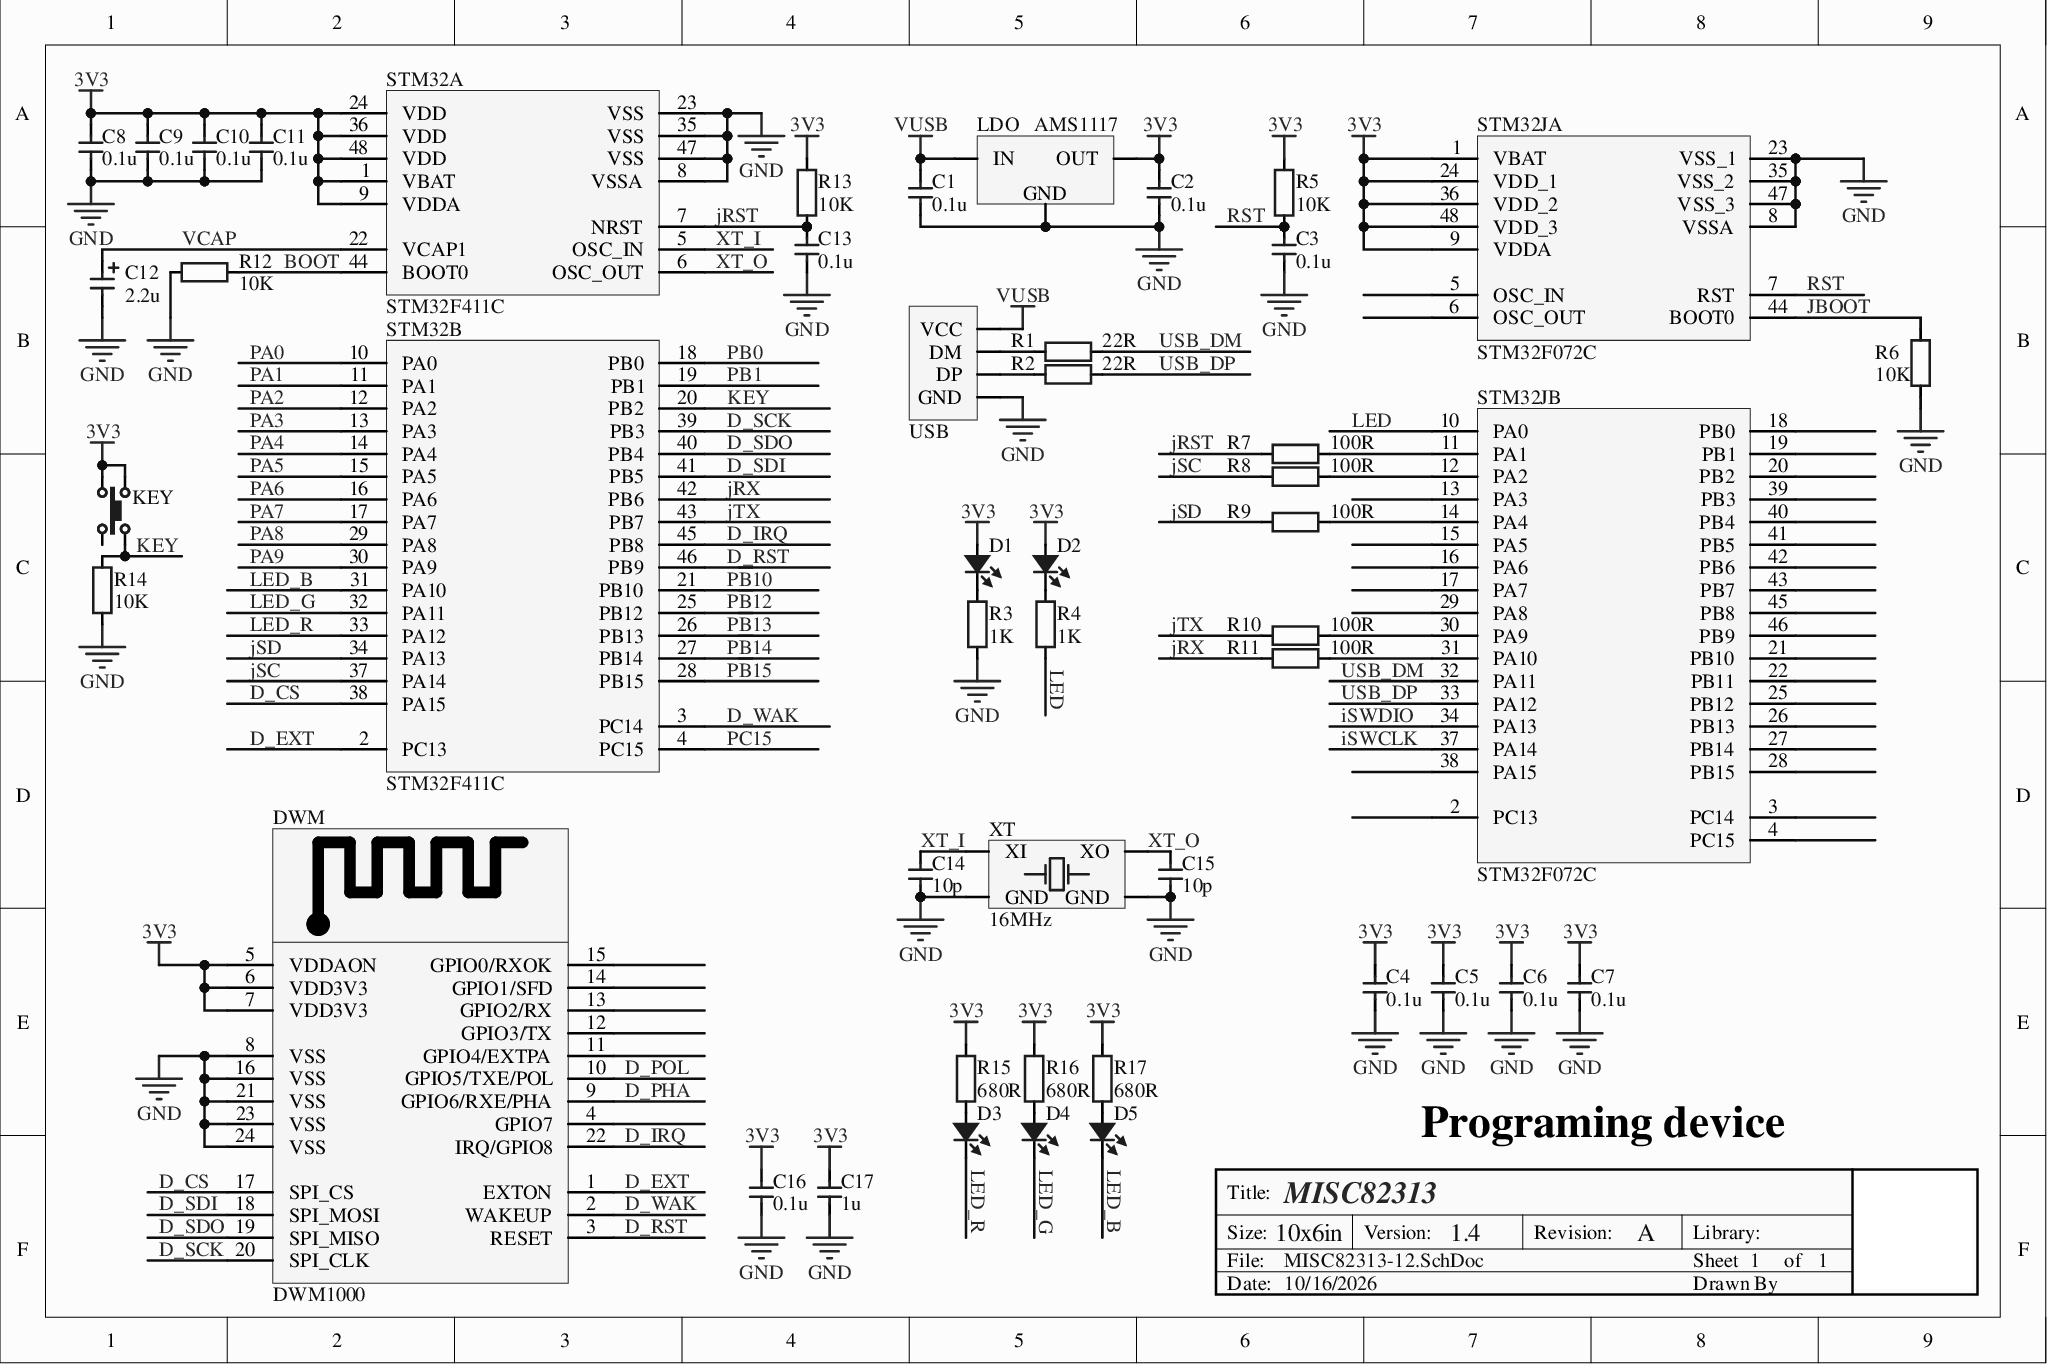
[diagram p0: MISC82313-12.SchDoc]
# Altium project MISC82313-6.PrjPCB
1 sheet, 46 parts. Net scope: global (net labels, ports and power ports of the same name join across sheets).
Board file: MISC82313-9.PcbDoc

## Sheet MISC82313-12.SchDoc: MISC82313
size 228 x 152 mm; Revision: A; SheetNumber: 1; SheetTotal: 1; Version: 1.4

### Parts
C1  value 0.1u  [CAP_0603]  (hidden comment: Cap_0603)
C2  value 0.1u  [CAP_0603]  (hidden comment: Cap_0603)
C3  value 0.1u  [CAP_0603]  (hidden comment: Cap_0603)
C4  value 0.1u  [CAP_0603]  (hidden comment: Cap_0603)
C5  value 0.1u  [CAP_0603]  (hidden comment: Cap_0603)
C6  value 0.1u  [CAP_0603]  (hidden comment: Cap_0603)
C7  value 0.1u  [CAP_0603]  (hidden comment: Cap_0603)
C8  value 0.1u  [CAP_0603]  (hidden comment: Cap_0603)
C9  value 0.1u  [CAP_0603]  (hidden comment: Cap_0603)
C10  value 0.1u  [CAP_0603]  (hidden comment: Cap_0603)
C11  value 0.1u  [CAP_0603]  (hidden comment: Cap_0603)
C12  value 2.2u  [CAP_TAN_P0805]  (hidden comment: Cap_Tan_0805)
C13  value 0.1u  [CAP_0603]  (hidden comment: Cap_0603)
C14  value 10p  [CAP_0603]  (hidden comment: Cap_0603)
C15  value 10p  [CAP_0603]  (hidden comment: Cap_0603)
C16  value 0.1u  [CAP_0603]  (hidden comment: Cap_0603)
C17  value 1u  [CAP_0603]  (hidden comment: Cap_0603)
D1  LED_0603  [LED_0603_YELLOW]  (value not drawn)
D2  LED_0603  [LED_0603_ORANGE]  (value not drawn)
D3  LED_0603  [LED_0603_RED]  (value not drawn)
D4  LED_0603  [LED_0603_GREEN]  (value not drawn)
D5  LED_0603  [LED_0603_BLUE]  (value not drawn)
DWM  DWM1000  [DWM1000]
KEY  ButtonTACT  [ButtonTACT_3.5*3.55_90]  (value not drawn)
LDO  AMS1117  [SOT89-3]
R1  value 22R  [RES_0603]  (hidden comment: Res_0603)
R2  value 22R  [RES_0603]  (hidden comment: Res_0603)
R3  value 1K  [RES_0603]  (hidden comment: Res_0603)
R4  value 1K  [RES_0603]  (hidden comment: Res_0603)
R5  value 10K  [RES_0603]  (hidden comment: Res_0603)
R6  value 10K  [RES_0603]  (hidden comment: Res_0603)
R7  value 100R  [RES_0603]  (hidden comment: Res_0603)
R8  value 100R  [RES_0603]  (hidden comment: Res_0603)
R9  value 100R  [RES_0603]  (hidden comment: Res_0603)
R10  value 100R  [RES_0603]  (hidden comment: Res_0603)
R11  value 100R  [RES_0603]  (hidden comment: Res_0603)
R12  value 10K  [RES_0603]  (hidden comment: Res_0603)
R13  value 10K  [RES_0603]  (hidden comment: Res_0603)
R14  value 10K  [RES_0603]  (hidden comment: Res_0603)
R15  value 680R  [RES_0603]  (hidden comment: Res_0603)
R16  value 680R  [RES_0603]  (hidden comment: Res_0603)
R17  value 680R  [RES_0603]  (hidden comment: Res_0603)
STM32  STM32F411C  [QFN_P0.5_48]  (parts A,B of 2)
STM32J  STM32F072C  [LQFP_P0.5_48]  (parts A,B of 2)
USB  USB_Plug_TypeA  [USB_Plug_TypeA]  (value not drawn)
XT  value 16MHz  [XT_2520_4]  (hidden comment: XTAL_2520_4P)

### Nets
3V3: C2.2 C4.2 C5.2 C6.2 C7.2 C8.2 C9.2 C10.2 C11.2 C16.1 C17.1 D1.1(A) D2.1(A) DWM.5(VDDAON) DWM.6(VDD3V3) DWM.7(VDD3V3) KEY.1 KEY.3 LDO.2(OUT) R5.2 R13.2 R15.2 R16.2 R17.2 STM32.1(VBAT) STM32.9(VDDA) STM32.24(VDD) STM32.36(VDD) STM32.48(VDD) STM32J.1(VBAT) STM32J.9(VDDA) STM32J.24(VDD_1) STM32J.36(VDD_2) STM32J.48(VDD_3)
GND: C1.1 C2.1 C3.1 C4.1 C5.1 C6.1 C7.1 C8.1 C9.1 C10.1 C11.1 C12.2 C13.1 C14.1 C15.1 C16.2 C17.2 DWM.8(VSS) DWM.16(VSS) DWM.21(VSS) DWM.23(VSS) DWM.24(VSS) LDO.1(GND) R3.1 R6.1 R12.2 R14.1 STM32.8(VSSA) STM32.23(VSS) STM32.35(VSS) STM32.47(VSS) STM32J.8(VSSA) STM32J.23(VSS_1) STM32J.35(VSS_2) STM32J.47(VSS_3) USB.4(GND) XT.2(GND) XT.4(GND)
VUSB: C1.2 LDO.3(IN) USB.1(VCC)
BOOT: R12.1 STM32.44(BOOT0)
D_CS: DWM.17(SPI_CS) STM32.38(PA15)
D_EXT: DWM.1(EXTON) STM32.2(PC13)
D_IRQ: DWM.22(IRQ/GPIO8) STM32.45(PB8)
D_PHA: DWM.9(GPIO6/RXE/PHA)
D_POL: DWM.10(GPIO5/TXE/POL)
D_RST: DWM.3(RESET) STM32.46(PB9)
D_SCK: DWM.20(SPI_CLK) STM32.39(PB3)
D_SDI: DWM.18(SPI_MOSI) STM32.41(PB5)
D_SDO: DWM.19(SPI_MISO) STM32.40(PB4)
D_WAK: DWM.2(WAKEUP) STM32.3(PC14)
iSWCLK: STM32J.37(PA14)
iSWDIO: STM32J.34(PA13)
JBOOT: R6.2 STM32J.44(BOOT0)
jRST: C13.2 R7.1 R13.1 STM32.7(NRST)
jRX: R11.1 STM32.42(PB6)
jSC: R8.1 STM32.37(PA14)
jSD: R9.1 STM32.34(PA13)
jTX: R10.1 STM32.43(PB7)
KEY: KEY.2 R14.2 STM32.20(PB2)
LED: R4.1 STM32J.10(PA0)
LED_B: D5.2(K) STM32.31(PA10)
LED_G: D4.2(K) STM32.32(PA11)
LED_R: D3.2(K) STM32.33(PA12)
PA0: STM32.10(PA0)
PA1: STM32.11(PA1)
PA2: STM32.12(PA2)
PA3: STM32.13(PA3)
PA4: STM32.14(PA4)
PA5: STM32.15(PA5)
PA6: STM32.16(PA6)
PA7: STM32.17(PA7)
PA8: STM32.29(PA8)
PA9: STM32.30(PA9)
PB0: STM32.18(PB0)
PB1: STM32.19(PB1)
P~{B}10: STM32.21(PB10)
P~{B}12: STM32.25(PB12)
P~{B}13: STM32.26(PB13)
P~{B}14: STM32.27(PB14)
P~{B}15: STM32.28(PB15)
PC15: STM32.4(PC15)
RST: C3.2 R5.1 STM32J.7(RST)
USB_DM: R1.2 STM32J.32(PA11)
USB_DP: R2.2 STM32J.33(PA12)
VCAP: C12.1 STM32.22(VCAP1)
XT_I: C14.2 STM32.5(OSC_IN) XT.1(XI)
XT_O: C15.2 STM32.6(OSC_OUT) XT.3(XO)
NetD1_2: D1.2(K) R3.2
NetD2_2: D2.2(K) R4.2
NetD3_1: D3.1(A) R15.1
NetD4_1: D4.1(A) R16.1
NetD5_1: D5.1(A) R17.1
NetR1_1: R1.1 USB.2(DM)
NetR2_1: R2.1 USB.3(DP)
NetR7_2: R7.2 STM32J.11(PA1)
NetR8_2: R8.2 STM32J.12(PA2)
NetR9_2: R9.2 STM32J.14(PA4)
NetR10_2: R10.2 STM32J.30(PA9)
NetR11_2: R11.2 STM32J.31(PA10)

Not connected (* = marked no-connect by the designer): DWM 4(GPIO7) 11(GPIO4/EXTPA) 12(GPIO3/TX) 13(GPIO2/RX) 14(GPIO1/SFD) 15(GPIO0/RXOK); KEY 4*; STM32J 2(PC13)* 3(PC14)* 4(PC15)* 5(OSC_IN)* 6(OSC_OUT)* 13(PA3)* 15(PA5)* 16(PA6)* 17(PA7)* 18(PB0)* 19(PB1)* 20(PB2)* 21(PB10)* 22(PB11)* 25(PB12)* 26(PB13)* 27(PB14)* 28(PB15)* 29(PA8)* 38(PA15)* 39(PB3)* 40(PB4)* 41(PB5)* 42(PB6)* 43(PB7)* 45(PB8)* 46(PB9)*

### Notes on the sheet
- Programing device
- Title:
- Size:
- Date:
- File:
- 10x6in
- Version:
- Revision:
- Sheet
- Drawn By
- Library:
- of

### Library data of the parts
C1-C11 C13-C17 = Cap_0603: Capacitor
C12 = Cap_Tan_0805: Capacitor
D1-D5 = LED_0603: LED
DWM = DWM1000: Module; Manufacturer: Decawave Limited; Frequency: 3.5GHz ~ 6.5GHz; Data Rate: 6.8Mbps; Serial Interfaces: SPI; Antenna Type: Integrated, Chip; Voltage - Supply: 2.8 V ~ 3.6 V; Current - Receiving: 64mA; Current - Transmitting: 31mA; Supplier 1: Digi-Key; Manufacturer Part Number: DWM1000; RoHS: RoHS Compliant; Category: RF/IF and RFID; Stock 1: 1028; Pricing 1: 1=32.16, 10=26.704, 100=24.24, 250=22.51296 (USD); Packaging: Cut Tape (CT); RF Family/Standard: 802.15.4; Protocol: -; Modulation: -; Power - Output: -; Sensitivity: -; Memory Size: -; Mounting Type: Surface Mount; Operating Temperature: -40¢XC ~ 85¢XC; Package / Case: Module; ComponentLink1URL: http://www.decawave.com/sites/default/files/product-pdf/dwm1000-product-brief.pdf; ComponentLink1Description: http://www.decawave.com/sites/default/files/product-pdf/dwm1000-product-brief.pdf; Supplier Part Number 1: 1479-1002-1-ND
KEY = ButtonTACT: Button
LDO = LDO1117: Power
R1-R17 = Res_0603: Resistor
STM32 = STM32F4x1C: MCU
STM32J = STM32F103C: MCU
USB = USB_Plug_TypeA: USB
XT = XTAL_2520_4P: Crystal Oscillator